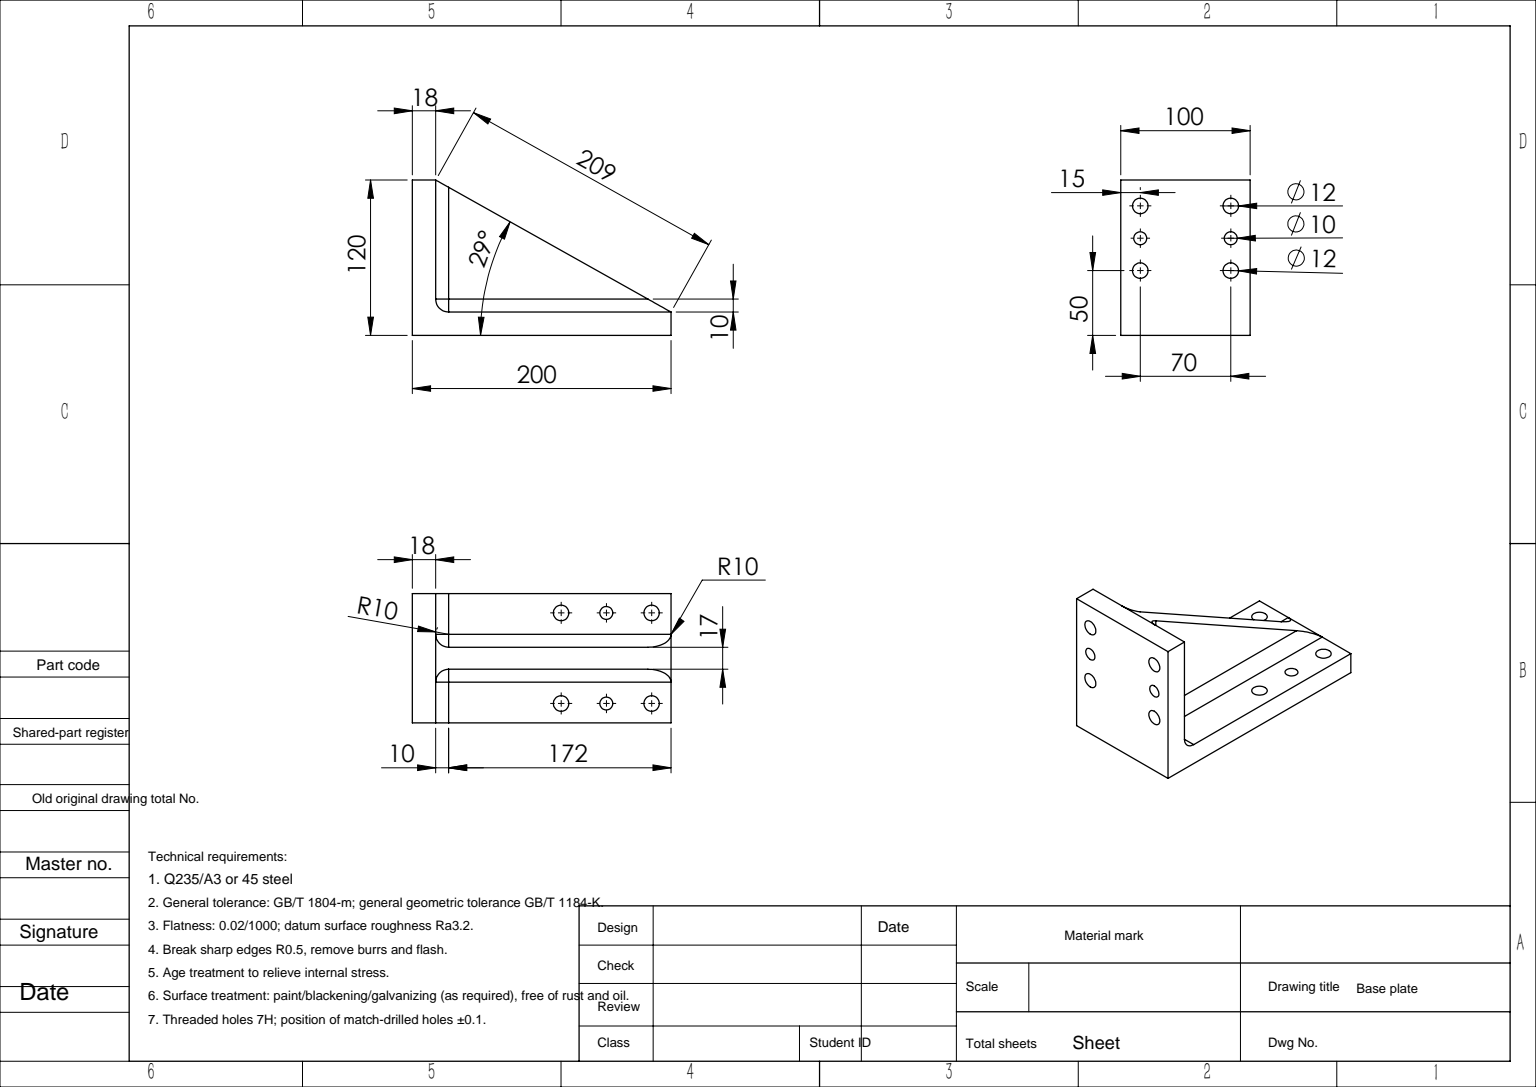
from build123d import *

# Parameters (mm, degrees)
BOSS_EXTRUDE1_DEPTH = 100
FILLET1_R           = 10
RIB3_REACH          = 240.537
SKETCH2_WALL_W      = 687.708067886
SKETCH2_WALL_H      = 17
FILLET2_R           = 10
SKETCH3_R           = 6
SKETCH3_R_2         = 5
CUT_EXTRUDE2_DEPTH  = 254.771550809
SKETCH7_R           = 6
SKETCH7_R_2         = 5
CUT_EXTRUDE3_DEPTH  = 254.771550809


with BuildPart() as part:
    # Sketch1 → Boss-Extrude1 (new body)
    with BuildSketch(Plane(origin=(0, 0, 0), x_dir=(0, 0, -1), z_dir=(1, 0, 0))):
        Polygon((0, 0), (0, 200), (120, 200), (120, 182), (18, 182), (18, 0), align=None)
    extrude(amount=BOSS_EXTRUDE1_DEPTH)

    # Fillet1
    fillet1_edges = [part.edges().sort_by_distance(p)[0] for p in [
        (50, 182, -18),
    ]]
    fillet(fillet1_edges, radius=FILLET1_R)

    # Sketch2 wall → Rib3 (add, up to next)
    with BuildSketch(Plane(origin=(50, 91, -69), x_dir=(0, -0.87234249996, 0.48889524723), z_dir=(0, -0.48889524723, -0.87234249996)), mode=Mode.PRIVATE) as rib3_sk1:
        Rectangle(SKETCH2_WALL_W, SKETCH2_WALL_H)
    rib3_tool1 = extrude(rib3_sk1.sketch, amount=-RIB3_REACH, mode=Mode.PRIVATE) - part.part
    add(rib3_tool1.solids().sort_by_distance((50, 91, -69))[0])

    # Fillet2
    fillet2_edges = [part.edges().sort_by_distance(p)[0] for p in [
        (41.5, 179.071067812, -20.928932188),
        (58.5, 179.071067812, -20.928932188),
        (41.5, 86, -18),
        (41.5, 182, -74),
        (58.5, 182, -74),
        (58.5, 86, -18),
    ]]
    fillet(fillet2_edges, radius=FILLET2_R)

    # Sketch3 → Cut-Extrude2 (cut, through all)
    with BuildSketch(Plane.XY):
        with Locations((15, 15)):
            Circle(SKETCH3_R)
        with Locations((15, 50)):
            Circle(SKETCH3_R_2)
        with Locations((15, 85)):
            Circle(SKETCH3_R)
        with Locations(Location((85, 15, 0), (0, 0, 270))):
            Circle(SKETCH3_R)
        with Locations(Location((85, 50, 0), (0, 0, 270))):
            Circle(SKETCH3_R_2)
        with Locations(Location((85, 85, 0), (0, 0, 270))):
            Circle(SKETCH3_R)
    extrude(amount=-CUT_EXTRUDE2_DEPTH, mode=Mode.SUBTRACT)

    # Sketch7 → Cut-Extrude3 (cut, through all)
    with BuildSketch(Plane(origin=(0, 200, 0), x_dir=(1, 0, 0), z_dir=(0, 1, 0))):
        with Locations(Location((15, 100, 0), (0, 0, 270))):
            Circle(SKETCH7_R)
        with Locations(Location((15, 75, 0), (0, 0, 270))):
            Circle(SKETCH7_R_2)
        with Locations(Location((15, 50, 0), (0, 0, 270))):
            Circle(SKETCH7_R)
        with Locations(Location((85, 50, 0), (0, 0, 270))):
            Circle(SKETCH7_R)
        with Locations(Location((85, 75, 0), (0, 0, 270))):
            Circle(SKETCH7_R_2)
        with Locations(Location((85, 100, 0), (0, 0, 270))):
            Circle(SKETCH7_R)
    extrude(amount=-CUT_EXTRUDE3_DEPTH, mode=Mode.SUBTRACT)


solid = part.part
